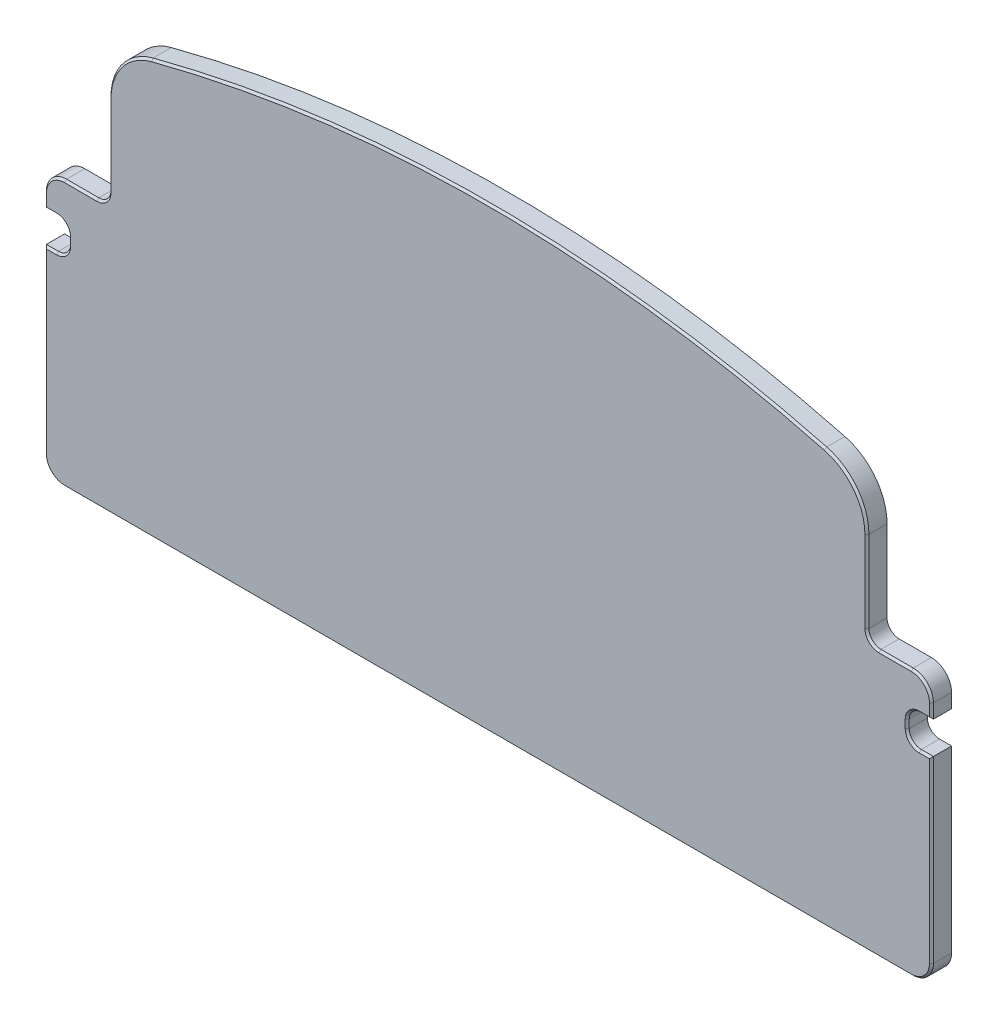
from build123d import *

# Parameters (mm, degrees)
SKETCH_1_W          = 220
SKETCH_1_H          = 121
EXTRUDE_1_DEPTH     = 2.5
CUT_EXTRUDE_1_DEPTH = 164.603178453
SKETCH_5_W          = 6
SKETCH_5_H          = 8
CUT_EXTRUDE_2_DEPTH = 159.13680786
FILLET_1_R          = 5
FILLET_2_R          = 3
CHAMFER_1_SIZE      = 0.5


with BuildPart() as part:
    # 草图1 → 凸台-拉伸1 (new, symmetric)
    with BuildSketch(Plane.XY):
        with Locations((0, 60.5)):
            Rectangle(SKETCH_1_W, SKETCH_1_H)
    extrude(amount=EXTRUDE_1_DEPTH, both=True)

    # 草图4 → 切除-拉伸1 (cut, through all)
    with BuildSketch(Plane.XY.offset(2.5)):
        with BuildLine():
            Line((-94, 66), (-110, 66))
            Line((-110, 66), (-110, 125.2))
            Line((-110, 125.2), (110, 125.2))
            Line((110, 125.2), (110, 66))
            Line((110, 66), (94, 66))
            Line((94, 66), (94, 89.205740869))
            ThreePointArc((94, 89.205740869), (91.081973046, 97.760848899), (83.544303797, 102.749666097))
            ThreePointArc((83.544303797, 102.749666097), (0, 113.5), (-83.544303797, 102.749666097))
            ThreePointArc((-83.544303797, 102.749666097), (-91.081973046, 97.760848899), (-94, 89.205740869))
            Line((-94, 89.205740869), (-94, 66))
        make_face()
    extrude(amount=-CUT_EXTRUDE_1_DEPTH, mode=Mode.SUBTRACT)

    # 草图5 → 切除-拉伸2 (cut, through all)
    with BuildSketch(Plane.XY.offset(2.5)):
        with Locations((-107, 53.5)):
            Rectangle(SKETCH_5_W, SKETCH_5_H)
        with Locations((107, 53.5)):
            Rectangle(SKETCH_5_W, SKETCH_5_H)
    extrude(amount=-CUT_EXTRUDE_2_DEPTH, mode=Mode.SUBTRACT)

    # 圆角1
    fillet_1_edges = [part.edges().sort_by_distance(p)[0] for p in [
        (-110, 66, 0),
        (110, 66, 0),
        (110, 0, 0),
        (-110, 0, 0),
    ]]
    fillet(fillet_1_edges, radius=FILLET_1_R)

    # 圆角2
    fillet_2_edges = [part.edges().sort_by_distance(p)[0] for p in [
        (-94, 66, 0),
        (94, 66, 0),
        (-104, 57.5, 0),
        (-104, 49.5, 0),
        (104, 49.5, 0),
        (104, 57.5, 0),
    ]]
    fillet(fillet_2_edges, radius=FILLET_2_R)

    # 倒角1
    chamfer_1_edges = [part.edges().sort_by_distance(p)[0] for p in [
        (-94, 79.102870434, 2.5),
        (101, 66, 2.5),
        (-104, 53.5, 2.5),
        (-108.5, 57.5, 2.5),
        (108.5, 49.5, 2.5),
        (104, 53.5, 2.5),
        (-94.878679656, 66.878679656, 2.5),
        (94.878679656, 66.878679656, 2.5),
        (-104.878679656, 50.378679656, 2.5),
        (-104.878679656, 56.621320344, 2.5),
        (104.878679656, 50.378679656, 2.5),
        (104.878679656, 56.621320344, 2.5),
        (-91.081973046, 97.760848899, 2.5),
        (0, 113.5, 2.5),
        (91.081973046, 97.760848899, 2.5),
        (94, 79.102870434, 2.5),
        (-110, 27.25, 2.5),
        (-108.5, 49.5, 2.5),
        (110, 59.25, 2.5),
        (108.5, 57.5, 2.5),
        (-101, 66, 2.5),
        (-110, 59.25, 2.5),
        (0, 0, 2.5),
        (110, 27.25, 2.5),
        (108.535533906, 1.464466094, 2.5),
        (-108.535533906, 1.464466094, 2.5),
        (108.535533906, 64.535533906, 2.5),
        (-108.535533906, 64.535533906, 2.5),
    ]]
    chamfer(chamfer_1_edges, length=CHAMFER_1_SIZE)


solid = part.part
